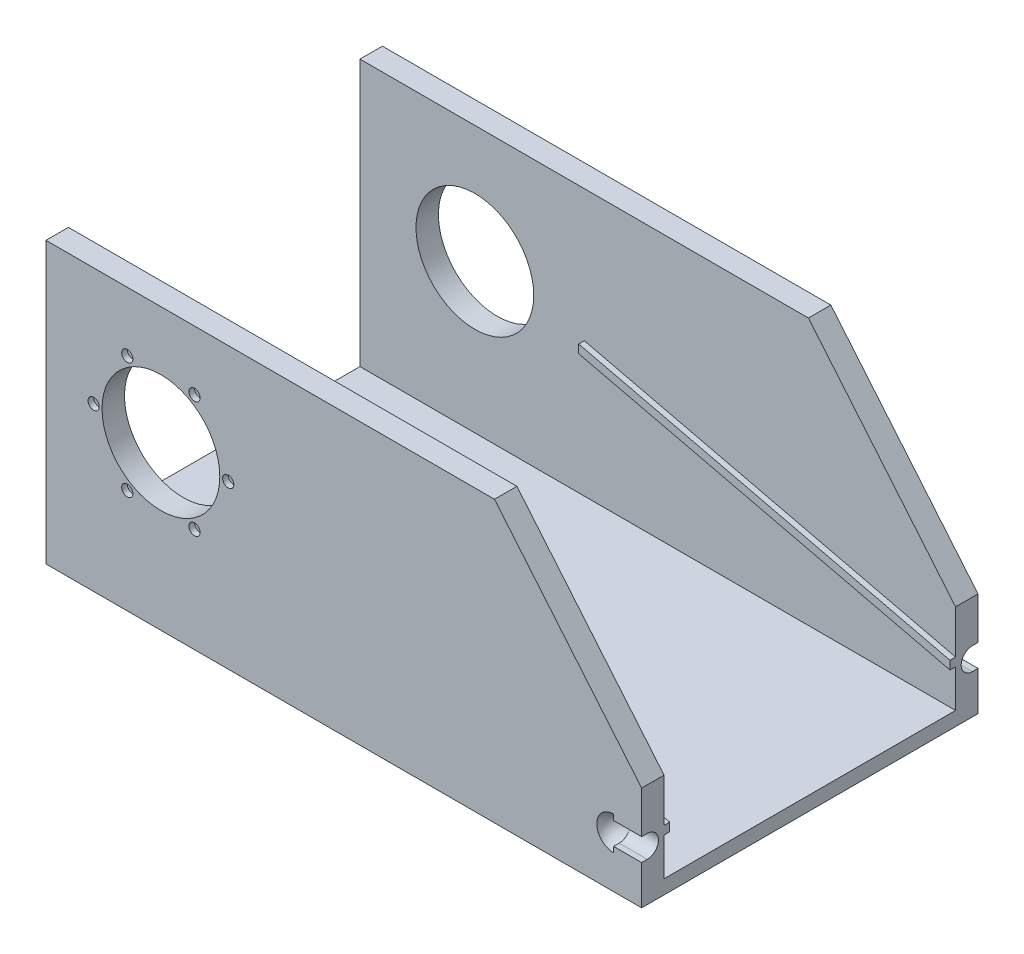
SolidWorks part; units mm, degrees
ref_plane "前视基准面" through (0, 0, 0) normal (0, 0, 1) x (1, 0, 0)
ref_plane "上视基准面" through (0, 0, 0) normal (0, 1, 0) x (1, 0, 0)
ref_plane "右视基准面" through (0, 0, 0) normal (1, 0, 0) x (0, 0, -1)
sketch "草图1" plane through (0, 0, 0) normal (0, 0, 1) x (1, 0, 0)
  line L0 (0, 0) -> (0, -1000)
  line L1 (0, -1000) -> (2125, -1000)
  line L2 (2125, -1000) -> (2125, -630)
  line L4 (0, 0) -> (1600, 0)
  line L7 (1600, 0) -> (2125, -630)
extrude "凸台-拉伸1" add sketch "草图1" along normal blind 80
sketch "草图4" plane through (0, 0, 0) normal (1, 0, 0) x (0, 0, -1)
  line L0 (-80, -1000) -> (-600, -1000)
  line L1 (-600, -1000) -> (-600, -950)
  line L2 (-600, -950) -> (-80, -950)
  line L3 (-80, 0) -> (-80, -1000) construction
  line L4 (-80, -950) -> (-80, -1000)
extrude "凸台-拉伸2" add sketch "草图4" along normal blind 2125
sketch3d "3D草图1"
  point P0 (1034.1875, -978.9898, 600)
ref_plane "基准面1" through (0, 0, 600) normal (0, 0, 1) x (1, 0, 0)
mirror "镜向4" about plane through (0, 0, 600) normal (0, 0, 1) of "凸台-拉伸2"
sketch3d "3D草图2"
  point P0 (1099.5118, -970.7155, 1120)
ref_plane "基准面2" through (0, 0, 1120) normal (0, 0, 1) x (1, 0, 0)
sketch "草图5" plane through (0, 0, 1120) normal (0, 0, 1) x (1, 0, 0)
  line L0 (0, -1000) -> (0, 0)
  line L1 (0, 0) -> (1600, 0)
  line L2 (1600, 0) -> (2125, -630)
  line L3 (2125, -630) -> (2125, -1000)
  line L4 (2125, -1000) -> (0, -1000)
extrude "凸台-拉伸3" add sketch "草图5" along normal blind 80
sketch "草图2" plane through (0, 0, 0) normal (0, 0, 1) x (1, 0, 0)
  circle A0 centre (410, -420) radius 210
extrude "切除-拉伸3" cut sketch "草图2" along normal through all both and the other way through all
sketch "草图6" plane through (0, 0, 0) normal (0, 0, 1) x (1, 0, 0)
  line L1 (800.5, -500) -> (2125, -815)
  line L2 (2125, -1000) -> (2125, -630) construction
  line L3 (2125, -815) -> (2125, -785)
  line L4 (2125, -785) -> (800.5, -470)
  line L5 (800.5, -470) -> (800.5, -500)
extrude "凸台-拉伸4" add sketch "草图6" along normal blind 100
mirror "镜向5" about plane through (0, 0, 600) normal (0, 0, 1) of "凸台-拉伸4"
sketch "草图7" plane through (0, 0, 0) normal (0, 0, 1) x (1, 0, 0)
  circle A2 centre (170, -420) radius 20
  circle A3 centre (290, -627.8461) radius 20
  circle A4 centre (530, -627.8461) radius 20
  circle A5 centre (650, -420) radius 20
  circle A6 centre (290, -212.1539) radius 20
  circle A7 centre (530, -212.1539) radius 20
extrude "切除-拉伸5" cut sketch "草图7" along normal blind 20
mirror "镜向6" about plane through (0, 0, 600) normal (0, 0, 1) of "切除-拉伸5"
sketch3d "3D草图3"
  point P0 (2125, -766.4546, 1180.0948)
ref_plane "基准面3" through (2125, 0, 0) normal (1, 0, 0) x (0, 0, -1)
sketch "草图8" plane through (2125, 0, 0) normal (1, 0, 0) x (0, 0, -1)
  line L1 (-1200, -1000) -> (-1200, -630) construction
  line L2 (-1200, -860) -> (-1180, -860)
  line L3 (-1180, -780) -> (-1200, -780)
  line L4 (-1200, -780) -> (-1200, -860)
  arc A0 (-1180, -860) -> (-1180, -780) centre (-1180, -820) ccw
extrude "切除-拉伸6" cut sketch "草图8" against normal blind 100
sketch3d "3D草图4"
  point P0 (1630.1321, -676.4796, 1200)
ref_plane "基准面4" through (0, 0, 1200) normal (0, 0, 1) x (1, 0, 0)
sketch "草图9" plane through (0, 0, 1200) normal (0, 0, 1) x (1, 0, 0)
  line L0 (2025, -780) -> (2025, -860) construction
  line L1 (2025, -760) -> (2025, -880)
  arc A0 (2025, -760) -> (2025, -880) centre (2025, -820) ccw
revolve "切除-旋转1" cut sketch "草图9" angle 90 about L1
mirror "镜向7" about plane through (0, 0, 600) normal (0, 0, 1) of "切除-拉伸6", "切除-旋转1"
